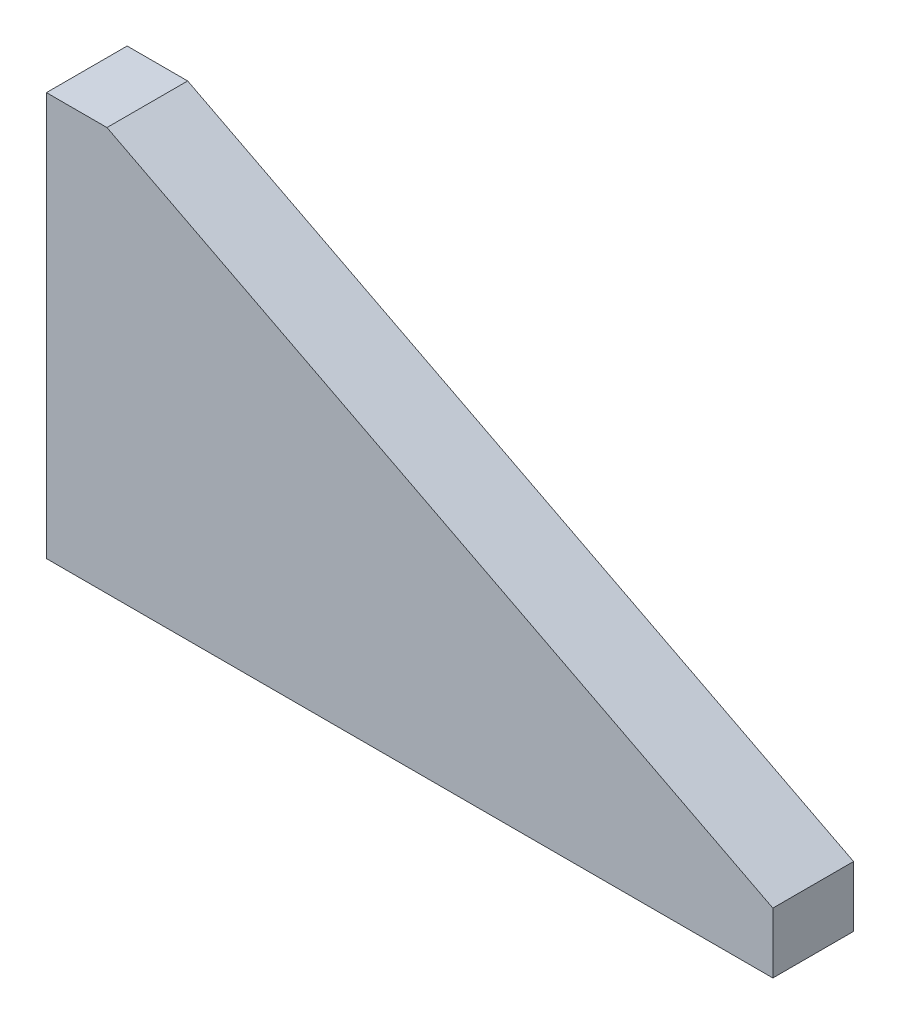
SolidWorks part; units mm, degrees
material "Q235B"
ref_plane "Front Plane" through (0, 0, 0) normal (0, 0, 1) x (1, 0, 0)
ref_plane "Top Plane" through (0, 0, 0) normal (0, 1, 0) x (1, 0, 0)
ref_plane "Right Plane" through (0, 0, 0) normal (1, 0, 0) x (0, 0, -1)
sketch "Sketch1" plane through (0, 0, 0) normal (0, 0, 1) x (1, 0, 0)
  line L0 (0, 0) -> (0, 100)
  line L1 (0, 100) -> (15, 100)
  line L2 (15, 100) -> (180, 15)
  line L3 (180, 15) -> (180, 0)
  line L4 (180, 0) -> (0, 0)
  dimension "D1" = 100
  dimension "D2" = 15
  dimension "D3" = 180
  dimension "D4" = 15
extrude "Boss-Extrude1" add sketch "Sketch1" along normal blind 20
